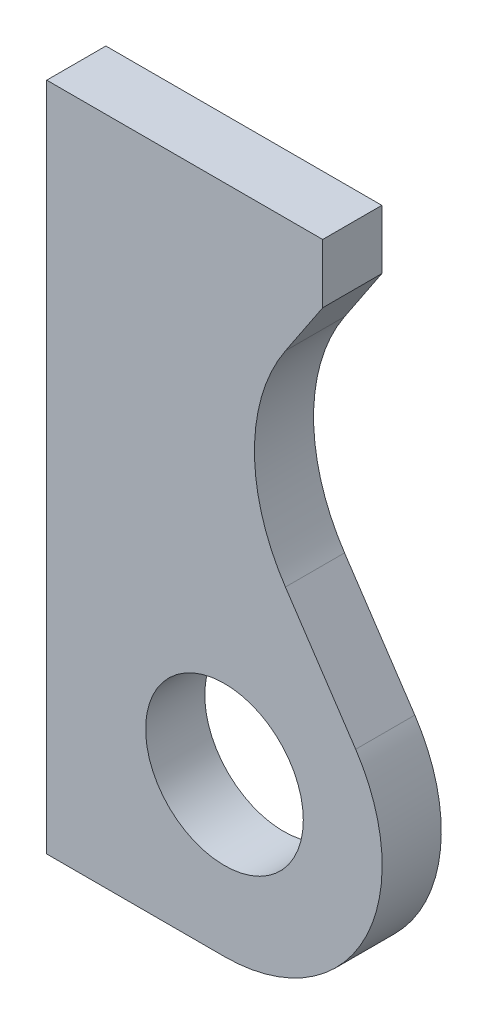
from build123d import *
from build123d.topology import SkipClean

# Parameters (mm, degrees)
SKETCH_1_R      = 20
EXTRUDE_1_DEPTH = 12
EXTRUDE_2_DEPTH = 10
EXTRUDE_3_DEPTH = 2
SKETCH_5_R      = 20
EXTRUDE_4_DEPTH = 3


with BuildPart() as part:
    # 草图1 → 凸台-拉伸1 (new body)
    with BuildSketch(Plane.XY):
        with BuildLine():
            Line((0, 0), (70, 0))
            Line((70, 0), (70, -15))
            Line((70, -15), (50, -45))
            Line((50, -45), (50, -65.266069056))
            Line((50, -65.266069056), (78.36394873, -107.811992151))
            ThreePointArc((78.36394873, -107.811992151), (80.348920907, -148.874317021), (45.081936956, -170))
            Line((45.081936956, -170), (0, -170))
            Line((0, -170), (0, 0))
        make_face()
        with Locations((45.081936956, -130)):
            Circle(SKETCH_1_R, mode=Mode.SUBTRACT)
    extrude(amount=EXTRUDE_1_DEPTH)

    # 草图3 → 凸台-拉伸2 (add)
    with BuildSketch(Plane.XY.offset(12)):
        with BuildLine():
            Line((50, -45), (50, -55.133034528))
            Line((50, -55.133034528), (52.687024396, -55.133034528))
            ThreePointArc((52.687024396, -55.133034528), (54.694220679, -41.57719354), (60.543560077, -29.184659884))
            Line((60.543560077, -29.184659884), (50, -45))
        make_face()
        with BuildLine():
            Line((52.687024396, -55.133034528), (50, -55.133034528))
            Line((50, -55.133034528), (50, -65.266069056))
            Line((50, -65.266069056), (60.543560077, -81.081409172))
            ThreePointArc((60.543560077, -81.081409172), (54.694220679, -68.688875516), (52.687024396, -55.133034528))
        make_face()
    extrude(amount=-EXTRUDE_2_DEPTH)

    # 草图4 → 凸台-拉伸3 (add)
    with BuildSketch(Plane(origin=(0, 0, 2), x_dir=(-1, 0, 0), z_dir=(0, 0, -1))):
        with BuildLine():
            Line((-60.543560077, -81.081409172), (-50, -65.266069056))
            Line((-50, -65.266069056), (-50, -45))
            Line((-50, -45), (-60.543560077, -29.184659884))
            ThreePointArc((-60.543560077, -29.184659884), (-52.687024396, -55.133034528), (-60.543560077, -81.081409172))
        make_face()
    extrude(amount=EXTRUDE_3_DEPTH)

    # 草图5 → 凸台-拉伸4 (add)
    with SkipClean():  # the faces are left unmerged after this step: merging them gives an invalid solid
        with BuildSketch(Plane.XY.offset(12)):
            with BuildLine():
                Line((0, 0), (0, -170))
                Line((0, -170), (45.081936956, -170))
                ThreePointArc((45.081936956, -170), (80.348920907, -148.874317021), (78.36394873, -107.811992151))
                Line((78.36394873, -107.811992151), (60.543560077, -81.081409172))
                ThreePointArc((60.543560077, -81.081409172), (52.687024396, -55.133034528), (60.543560077, -29.184659884))
                Line((60.543560077, -29.184659884), (70, -15))
                Line((70, -15), (70, 0))
                Line((70, 0), (0, 0))
            make_face()
            with Locations((45.081936956, -130)):
                Circle(SKETCH_5_R, mode=Mode.SUBTRACT)
        extrude(amount=EXTRUDE_4_DEPTH)


solid = part.part
